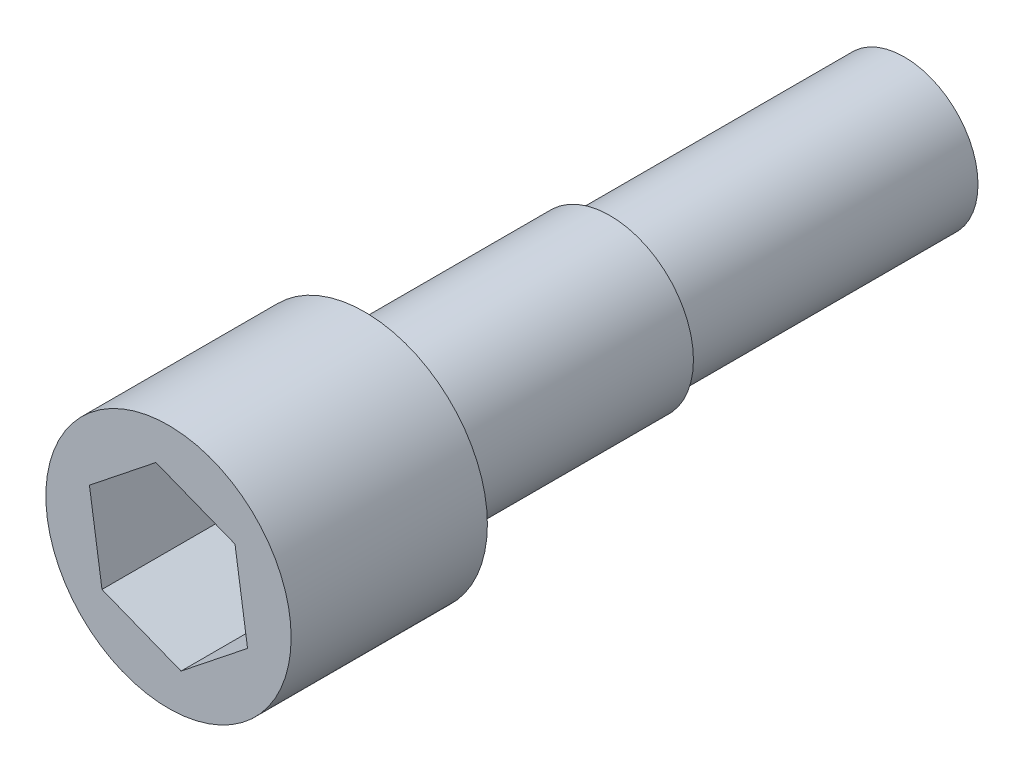
from build123d import *

# Parameters (mm, degrees)
SKETCH_1_R          = 1.7
EXTRUDE_1_DEPTH     = 5
SKETCH_2_R          = 1.5
EXTRUDE_2_DEPTH     = 6
SKETCH_3_R          = 2.5
EXTRUDE_3_DEPTH     = 4
CUT_EXTRUDE_1_DEPTH = 3


with BuildPart() as part:
    # 草图1 → 凸台-拉伸1 (new body)
    with BuildSketch(Plane.XY):
        with Locations((0, -6)):
            Circle(SKETCH_1_R)
    extrude(amount=-EXTRUDE_1_DEPTH)

    # 草图2 → 凸台-拉伸2 (add)
    with BuildSketch(Plane(origin=(0, 0, -5), x_dir=(-1, 0, 0), z_dir=(0, 0, -1))):
        with Locations(Location((0, -6, 0), (0, 0, 180))):
            Circle(SKETCH_2_R)
    extrude(amount=EXTRUDE_2_DEPTH)

    # 草图3 → 凸台-拉伸3 (add)
    with BuildSketch(Plane.XY):
        with Locations((0, -6)):
            Circle(SKETCH_3_R)
    extrude(amount=EXTRUDE_3_DEPTH)

    # 草图4 → 切除-拉伸1 (cut)
    with BuildSketch(Plane.XY.offset(4)):
        Polygon((1.355554736, -4.921820351), (-0.255953598, -4.286965337), (-1.611508335, -5.365144986), (-1.355554737, -7.078179649), (0.255953597, -7.713034663), (1.611508334, -6.634855014), align=None)
    extrude(amount=-CUT_EXTRUDE_1_DEPTH, mode=Mode.SUBTRACT)


solid = part.part
